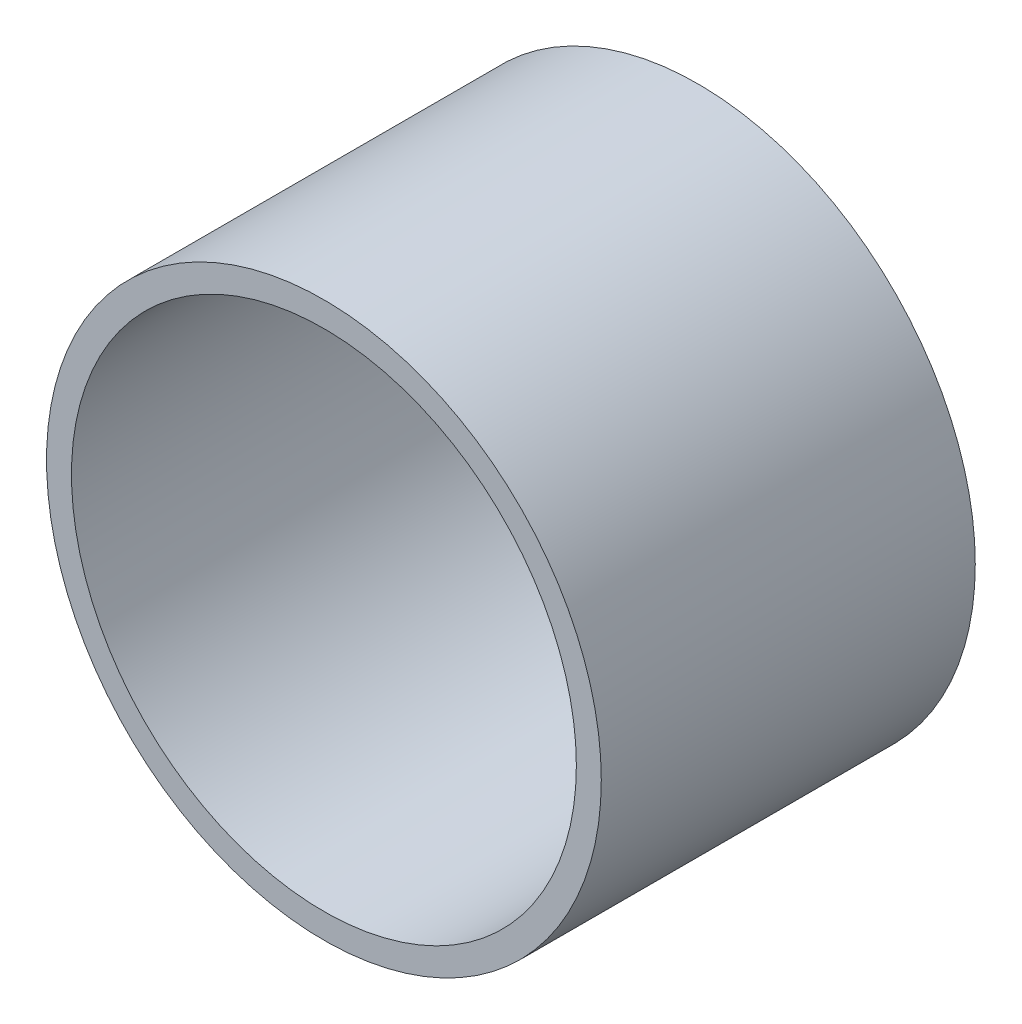
SolidWorks part; units mm, degrees
material "Q235B"
ref_plane "Front Plane" through (0, 0, 0) normal (0, 0, 1) x (1, 0, 0)
ref_plane "Top Plane" through (0, 0, 0) normal (0, 1, 0) x (1, 0, 0)
ref_plane "Right Plane" through (0, 0, 0) normal (1, 0, 0) x (0, 0, -1)
sketch "Sketch1" plane through (0, 0, 0) normal (0, 0, 1) x (1, 0, 0)
  circle A0 centre (-1060, 0) radius 44.5
  circle A1 centre (-1060, 0) radius 40.5
  dimension "D1" = 89
  dimension "D2" = 4
extrude "Boss-Extrude1" add sketch "Sketch1" along normal blind 60
